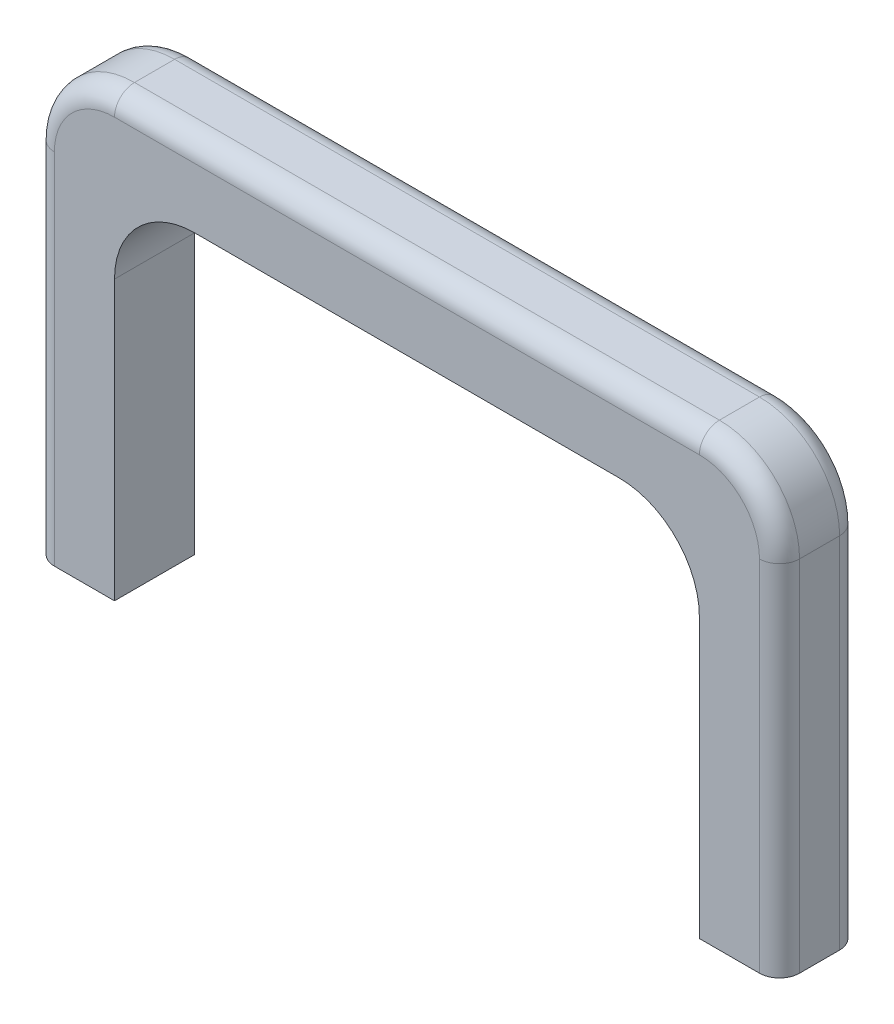
from build123d import *

# Parameters (mm, degrees)
EXTRUDE_THIN1_DEPTH = 2
FILLET1_R           = 2
FILLET2_R           = 0.5


with BuildPart() as part:
    # Sketch1 → Extrude-Thin1 (new body)
    with BuildSketch(Plane.XY):
        Polygon((0, 0), (0, 8.954475992), (14.596760519, 8.954475992), (14.596760519, 0), (16.596760519, 0), (16.596760519, 10.954475992), (-2, 10.954475992), (-2, 0), align=None)
    extrude(amount=EXTRUDE_THIN1_DEPTH)

    # Fillet1
    fillet1_edges = [part.edges().sort_by_distance(p)[0] for p in [
        (-2, 10.954475992, 1),
        (16.596760519, 10.954475992, 1),
        (14.596760519, 8.954475992, 1),
        (0, 8.954475992, 1),
    ]]
    fillet(fillet1_edges, radius=FILLET1_R)

    # Fillet2
    fillet2_edges = [part.edges().sort_by_distance(p)[0] for p in [
        (16.596760519, 4.477237996, 2),
        (7.29838026, 10.954475992, 0),
        (7.29838026, 10.954475992, 2),
        (-2, 4.477237996, 0),
        (-1.414213562, 10.368689555, 0),
        (16.010974082, 10.368689555, 0),
        (-2, 4.477237996, 2),
        (-1.414213562, 10.368689555, 2),
        (16.010974082, 10.368689555, 2),
        (16.596760519, 4.477237996, 0),
    ]]
    fillet(fillet2_edges, radius=FILLET2_R)


solid = part.part
